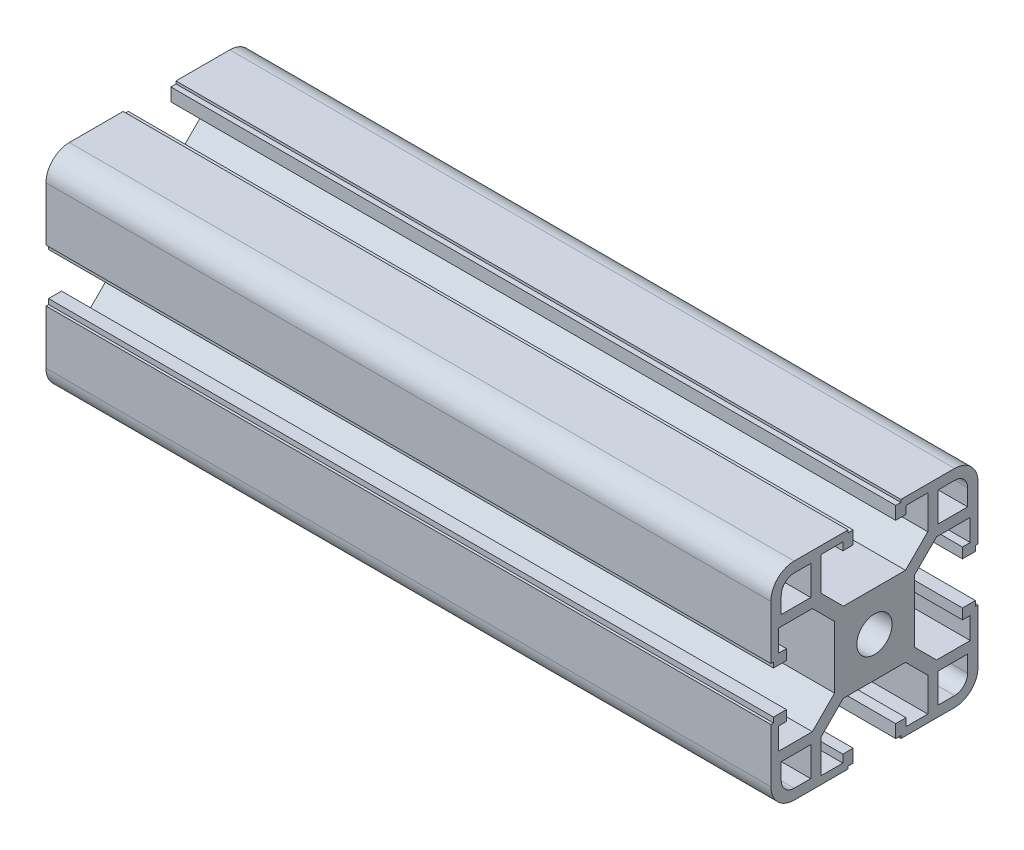
from build123d import *

# Parameters (mm, degrees)
SKETCH1_R                                 = 3.4
ALUMINIUM_PROFILE_40_X_40B_X_R4_5_1_DEPTH = 140


with BuildPart() as part:
    # Sketch1 → Aluminium profile 40 X 40B X R4.5(1) (new body)
    with BuildSketch(Plane.YZ.offset(-984.974958264)):
        with BuildLine():
            Line((-5.1, 20), (-5.1, 19.5))
            Line((-5.1, 19.5), (-4.1, 19.5))
            Line((-4.1, 19.5), (-4.1, 17))
            Line((-4.1, 17), (-6.1, 17))
            Line((-6.1, 17), (-6.1, 18.5))
            Line((-6.1, 18.5), (-10.3, 18.5))
            Line((-10.3, 18.5), (-10.3, 12))
            Line((-10.3, 12), (-6, 7.7))
            Line((-6, 7.7), (6, 7.7))
            Line((6, 7.7), (10.3, 12))
            Line((10.3, 12), (10.3, 18.5))
            Line((10.3, 18.5), (6.1, 18.5))
            Line((6.1, 18.5), (6.1, 17))
            Line((6.1, 17), (4.1, 17))
            Line((4.1, 17), (4.1, 19.5))
            Line((4.1, 19.5), (5.1, 19.5))
            Line((5.1, 19.5), (5.1, 20))
            Line((5.1, 20), (15.5, 20))
            ThreePointArc((15.5, 20), (18.681980515, 18.681980515), (20, 15.5))
            Line((20, 15.5), (20, 5.1))
            Line((20, 5.1), (19.5, 5.1))
            Line((19.5, 5.1), (19.5, 4.1))
            Line((19.5, 4.1), (17, 4.1))
            Line((17, 4.1), (17, 6.1))
            Line((17, 6.1), (18.5, 6.1))
            Line((18.5, 6.1), (18.5, 10.3))
            Line((18.5, 10.3), (12, 10.3))
            Line((12, 10.3), (7.7, 6))
            Line((7.7, 6), (7.7, -6))
            Line((7.7, -6), (12, -10.3))
            Line((12, -10.3), (18.5, -10.3))
            Line((18.5, -10.3), (18.5, -6.1))
            Line((18.5, -6.1), (17, -6.1))
            Line((17, -6.1), (17, -4.1))
            Line((17, -4.1), (19.5, -4.1))
            Line((19.5, -4.1), (19.5, -5.1))
            Line((19.5, -5.1), (20, -5.1))
            Line((20, -5.1), (20, -15.5))
            ThreePointArc((20, -15.5), (18.681980515, -18.681980515), (15.5, -20))
            Line((15.5, -20), (5.1, -20))
            Line((5.1, -20), (5.1, -19.5))
            Line((5.1, -19.5), (4.1, -19.5))
            Line((4.1, -19.5), (4.1, -17))
            Line((4.1, -17), (6.1, -17))
            Line((6.1, -17), (6.1, -18.5))
            Line((6.1, -18.5), (10.3, -18.5))
            Line((10.3, -18.5), (10.3, -12))
            Line((10.3, -12), (6, -7.7))
            Line((6, -7.7), (-6, -7.7))
            Line((-6, -7.7), (-10.3, -12))
            Line((-10.3, -12), (-10.3, -18.5))
            Line((-10.3, -18.5), (-6.1, -18.5))
            Line((-6.1, -18.5), (-6.1, -17))
            Line((-6.1, -17), (-4.1, -17))
            Line((-4.1, -17), (-4.1, -19.5))
            Line((-4.1, -19.5), (-5.1, -19.5))
            Line((-5.1, -19.5), (-5.1, -20))
            Line((-5.1, -20), (-15.5, -20))
            ThreePointArc((-15.5, -20), (-18.681980515, -18.681980515), (-20, -15.5))
            Line((-20, -15.5), (-20, -5.1))
            Line((-20, -5.1), (-19.5, -5.1))
            Line((-19.5, -5.1), (-19.5, -4.1))
            Line((-19.5, -4.1), (-17, -4.1))
            Line((-17, -4.1), (-17, -6.1))
            Line((-17, -6.1), (-18.5, -6.1))
            Line((-18.5, -6.1), (-18.5, -10.3))
            Line((-18.5, -10.3), (-12, -10.3))
            Line((-12, -10.3), (-7.7, -6))
            Line((-7.7, -6), (-7.7, 6))
            Line((-7.7, 6), (-12, 10.3))
            Line((-12, 10.3), (-18.5, 10.3))
            Line((-18.5, 10.3), (-18.5, 6.1))
            Line((-18.5, 6.1), (-17, 6.1))
            Line((-17, 6.1), (-17, 4.1))
            Line((-17, 4.1), (-19.5, 4.1))
            Line((-19.5, 4.1), (-19.5, 5.1))
            Line((-19.5, 5.1), (-20, 5.1))
            Line((-20, 5.1), (-20, 15.5))
            ThreePointArc((-20, 15.5), (-18.681980515, 18.681980515), (-15.5, 20))
            Line((-15.5, 20), (-5.1, 20))
        make_face()
        Circle(SKETCH1_R, mode=Mode.SUBTRACT)
        with BuildLine():
            Line((12.3, 18), (15.5, 18))
            ThreePointArc((15.5, 18), (17.267766953, 17.267766953), (18, 15.5))
            Line((18, 15.5), (18, 12.3))
            Line((18, 12.3), (12.3, 12.3))
            Line((12.3, 12.3), (12.3, 18))
        make_face(mode=Mode.SUBTRACT)
        with BuildLine():
            Line((-15.5, 18), (-12.3, 18))
            Line((-12.3, 18), (-12.3, 12.3))
            Line((-12.3, 12.3), (-18, 12.3))
            Line((-18, 12.3), (-18, 15.5))
            ThreePointArc((-18, 15.5), (-17.267766953, 17.267766953), (-15.5, 18))
        make_face(mode=Mode.SUBTRACT)
        with BuildLine():
            Line((-18, -12.3), (-12.3, -12.3))
            Line((-12.3, -12.3), (-12.3, -18))
            Line((-12.3, -18), (-15.5, -18))
            ThreePointArc((-15.5, -18), (-17.267766953, -17.267766953), (-18, -15.5))
            Line((-18, -15.5), (-18, -12.3))
        make_face(mode=Mode.SUBTRACT)
        with BuildLine():
            Line((12.3, -12.3), (18, -12.3))
            Line((18, -12.3), (18, -15.5))
            ThreePointArc((18, -15.5), (17.267766953, -17.267766953), (15.5, -18))
            Line((15.5, -18), (12.3, -18))
            Line((12.3, -18), (12.3, -12.3))
        make_face(mode=Mode.SUBTRACT)
    extrude(amount=ALUMINIUM_PROFILE_40_X_40B_X_R4_5_1_DEPTH)


solid = part.part
